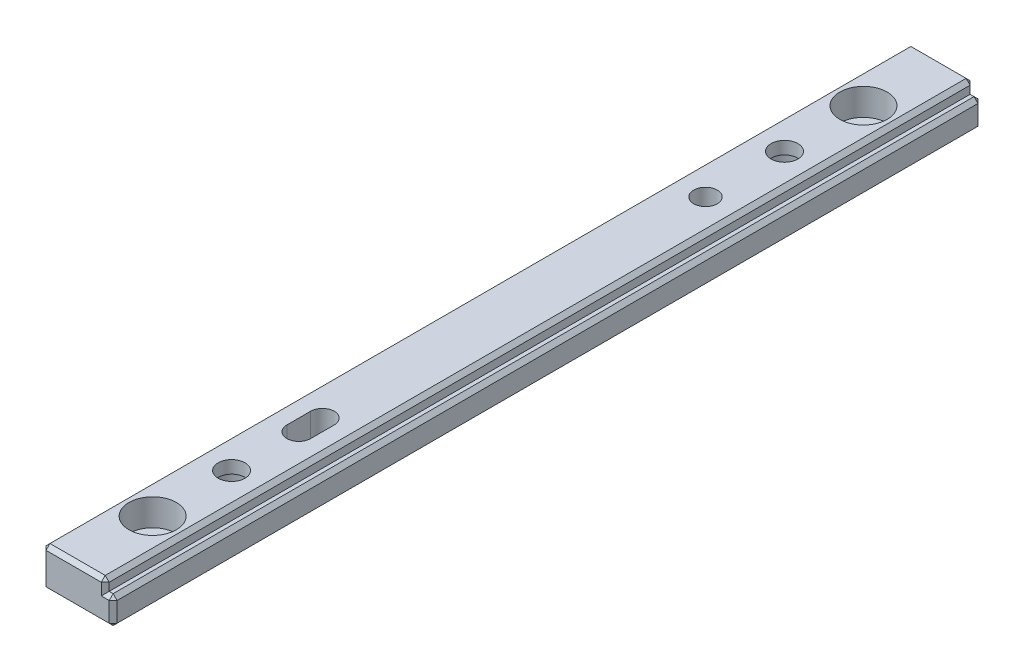
from build123d import *

# Parameters (mm, degrees)
BOSS_EXTRUDE2_DEPTH                                  = 110
CBORE_FOR_M3_SLOTTED_CHEESE_HEAD_SCREWS2_D           = 3.4
CBORE_FOR_M3_SLOTTED_CHEESE_HEAD_SCREWS2_CBORE_D     = 6
CBORE_FOR_M3_SLOTTED_CHEESE_HEAD_SCREWS2_CBORE_DEPTH = 3.4
CBORE_FOR_M3_SLOTTED_CHEESE_HEAD_SCREWS3_D           = 3.4
CBORE_FOR_M3_SLOTTED_CHEESE_HEAD_SCREWS3_CBORE_D     = 6
CBORE_FOR_M3_SLOTTED_CHEESE_HEAD_SCREWS3_CBORE_DEPTH = 3.4
F_3_0MM_DOWEL_HOLE1_D                                = 3
CUT_EXTRUDE1_DEPTH                                   = 111.480767557
CHAMFER1_SIZE                                        = 0.5


with BuildPart() as part:
    # Sketch4 → Boss-Extrude2 (new body)
    with BuildSketch(Plane.XY):
        Polygon((0, 0), (9, 0), (9, 3.5), (8, 3.5), (8, 5), (0, 5), (0, 3.5), align=None)
    extrude(amount=BOSS_EXTRUDE2_DEPTH)

    # CBORE for M3 Slotted cheese head screws2 (through all)
    with Locations(Plane(origin=(0, 5, 0), x_dir=(1, 0, 0), z_dir=(0, 1, 0))):
        with Locations((4, -10), (4, -100)):
            CounterBoreHole(CBORE_FOR_M3_SLOTTED_CHEESE_HEAD_SCREWS2_D / 2, CBORE_FOR_M3_SLOTTED_CHEESE_HEAD_SCREWS2_CBORE_D / 2, CBORE_FOR_M3_SLOTTED_CHEESE_HEAD_SCREWS2_CBORE_DEPTH)

    # CBORE for M3 Slotted cheese head screws3 (through all)
    with Locations(Plane.XZ):
        with Locations((4, 90), (4, 20)):
            CounterBoreHole(CBORE_FOR_M3_SLOTTED_CHEESE_HEAD_SCREWS3_D / 2, CBORE_FOR_M3_SLOTTED_CHEESE_HEAD_SCREWS3_CBORE_D / 2, CBORE_FOR_M3_SLOTTED_CHEESE_HEAD_SCREWS3_CBORE_DEPTH)

    # Ø3.0mm dowel hole1 (through all)
    with Locations(Plane.XZ):
        with Locations((4, 80), (4, 30)):
            Hole(F_3_0MM_DOWEL_HOLE1_D / 2)

    # Sketch11 → Cut-Extrude1 (cut, through all)
    with BuildSketch(Plane.XZ):
        with BuildLine():
            Line((2.5, 78.5), (2.5, 81.5))
            ThreePointArc((2.5, 81.5), (4, 83), (5.5, 81.5))
            Line((5.5, 81.5), (5.5, 78.5))
            ThreePointArc((5.5, 78.5), (4, 77), (2.5, 78.5))
        make_face()
    extrude(amount=-CUT_EXTRUDE1_DEPTH, mode=Mode.SUBTRACT)

    # Chamfer1
    chamfer1_edges = [part.edges().sort_by_distance(p)[0] for p in [
        (0, 5, 55),
        (8, 5, 55),
        (9, 1.75, 110),
        (9, 3.5, 55),
        (9, 0, 55),
        (0, 0, 55),
        (8.5, 3.5, 110),
        (8, 4.25, 110),
        (4, 5, 110),
        (0, 2.5, 110),
        (0, 2.5, 0),
        (4, 5, 0),
        (8, 4.25, 0),
        (8.5, 3.5, 0),
        (4.5, 0, 110),
        (9, 1.75, 0),
        (4.5, 0, 0),
    ]]
    chamfer(chamfer1_edges, length=CHAMFER1_SIZE)


solid = part.part
